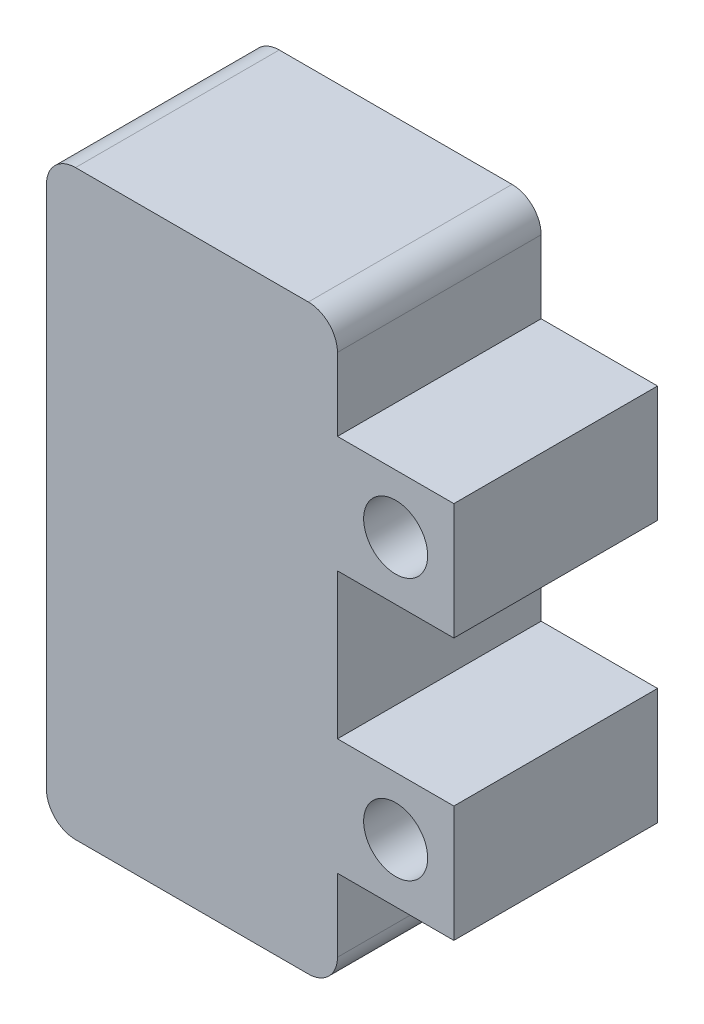
from build123d import *

# Parameters (mm, degrees)
SKETCH_1_W          = 10
SKETCH_1_H          = 20
EXTRUDE_1_DEPTH     = 7
SKETCH_2_W          = 4
SKETCH_2_H          = 4
SKETCH_2_R          = 1.1
EXTRUDE_2_DEPTH     = 7
FILLET_1_R          = 1
SKETCH_3_W          = 5.954377652
SKETCH_3_H          = 2.653951182
CUT_EXTRUDE_1_DEPTH = 0.1


with BuildPart() as part:
    # 草图1 → 凸台-拉伸1 (new body)
    with BuildSketch(Plane.XY):
        Rectangle(SKETCH_1_W, SKETCH_1_H)
    extrude(amount=EXTRUDE_1_DEPTH)

    # 草图2 → 凸台-拉伸2 (add)
    # profile 1 of 2: a face of its own
    with BuildSketch(Plane.XY.offset(7)):
        with Locations((7, 4.5)):
            Rectangle(SKETCH_2_W, SKETCH_2_H)
        with Locations((7, 4.5)):
            Circle(SKETCH_2_R, mode=Mode.SUBTRACT)
    # profile 2 of 2: a face of its own
    with BuildSketch(Plane.XY.offset(7)):
        with Locations((7, -4.5)):
            Rectangle(SKETCH_2_W, SKETCH_2_H)
        with Locations((7, -4.5)):
            Circle(SKETCH_2_R, mode=Mode.SUBTRACT)
    extrude(amount=-EXTRUDE_2_DEPTH)

    # 圆角1
    fillet_1_edges = [part.edges().sort_by_distance(p)[0] for p in [
        (5, -10, 3.5),
        (-5, -10, 3.5),
        (5, 10, 3.5),
        (-5, 10, 3.5),
    ]]
    fillet(fillet_1_edges, radius=FILLET_1_R)

    # 草图3 → 切除-拉伸1 (cut)
    with BuildSketch(Plane.ZY.offset(5)):
        with Locations((3.551037523, 7.111228168)):
            Rectangle(SKETCH_3_W, SKETCH_3_H)
    cut_extrude_1 = extrude(amount=-CUT_EXTRUDE_1_DEPTH, mode=Mode.SUBTRACT)

    # 镜向1: 切除-拉伸1 across plane
    add(cut_extrude_1.mirror(Plane.ZX), mode=Mode.SUBTRACT)


solid = part.part
